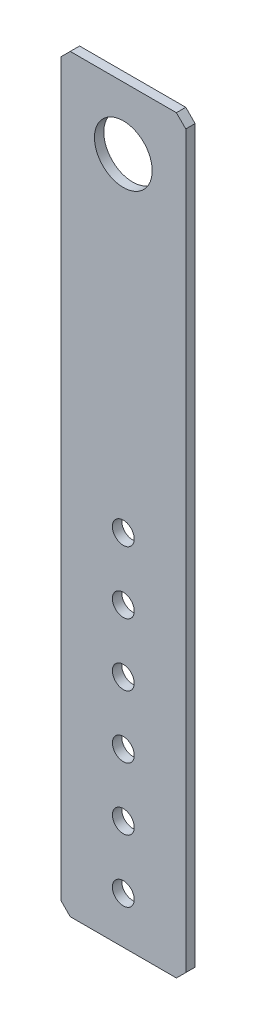
from build123d import *

# Parameters (mm, degrees)
SKETCH1_R           = 9.25
SKETCH1_R_2         = 3.5
BOSS_EXTRUDE1_DEPTH = 1.5


with BuildPart() as part:
    # Sketch1 → Boss-Extrude1 (new, symmetric)
    with BuildSketch(Plane.XY):
        Polygon((-20, 117), (-17, 120), (17, 120), (20, 117), (20, -117), (17, -120), (-17, -120), (-20, -117), align=None)
        with Locations((0, 100)):
            Circle(SKETCH1_R, mode=Mode.SUBTRACT)
        with Locations((0, -105)):
            Circle(SKETCH1_R_2, mode=Mode.SUBTRACT)
        with Locations((0, -85)):
            Circle(SKETCH1_R_2, mode=Mode.SUBTRACT)
        with Locations((0, -65)):
            Circle(SKETCH1_R_2, mode=Mode.SUBTRACT)
        with Locations((0, -45)):
            Circle(SKETCH1_R_2, mode=Mode.SUBTRACT)
        with Locations((0, -25)):
            Circle(SKETCH1_R_2, mode=Mode.SUBTRACT)
        with Locations((0, -5)):
            Circle(SKETCH1_R_2, mode=Mode.SUBTRACT)
    extrude(amount=BOSS_EXTRUDE1_DEPTH, both=True)


solid = part.part
